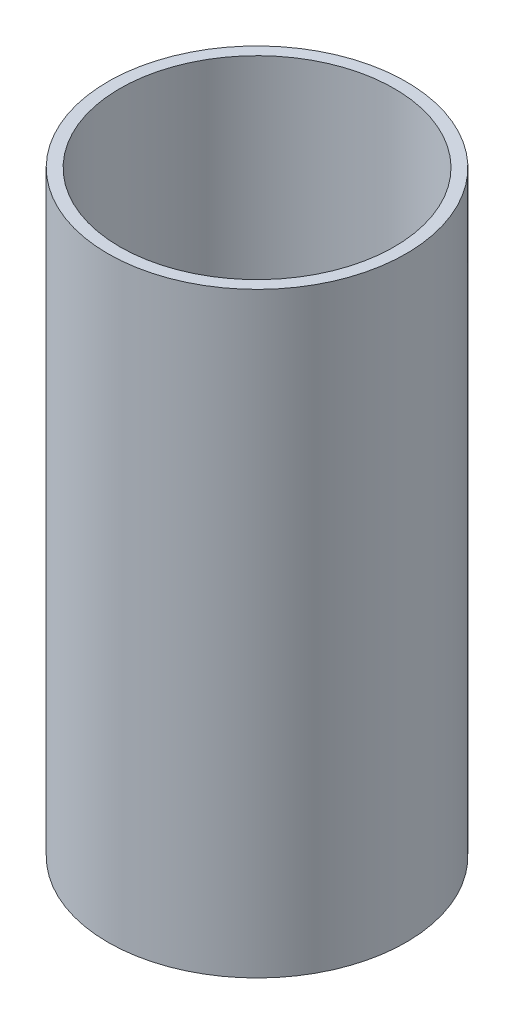
SolidWorks part; units mm, degrees
material "Q235B"
ref_plane "Front Plane" through (0, 0, 0) normal (0, 0, 1) x (1, 0, 0)
ref_plane "Top Plane" through (0, 0, 0) normal (0, 1, 0) x (1, 0, 0)
ref_plane "Right Plane" through (0, 0, 0) normal (1, 0, 0) x (0, 0, -1)
sketch "Sketch1" plane through (0, 0, 0) normal (0, 1, 0) x (1, 0, 0)
  circle A0 centre (0, 0) radius 25
  circle A1 centre (0, 0) radius 23
  dimension "D1" = 50
  dimension "D2" = 2
extrude "Boss-Extrude1" add sketch "Sketch1" along normal blind 100
sketch "Sketch2" plane through (0, 0, 0) normal (0, 0, 1) x (1, 0, 0)
  line L0 (0, 0) -> (0, 40) construction
  line L1 (-25, 0) -> (25, 0) construction
  line L2 (-20, 0) -> (-20, 40)
  line L3 (20, 0) -> (20, 40)
  arc A0 (-20, 0) -> (20, 0) centre (0, 0) ccw
  arc A1 (20, 40) -> (-20, 40) centre (0, 40) ccw
  point P4 (0, 20)
  dimension "D2" = 20
  dimension "D1" = 40
extrude "Cut-Extrude1" [suppressed] cut sketch "Sketch2" along normal up to next
